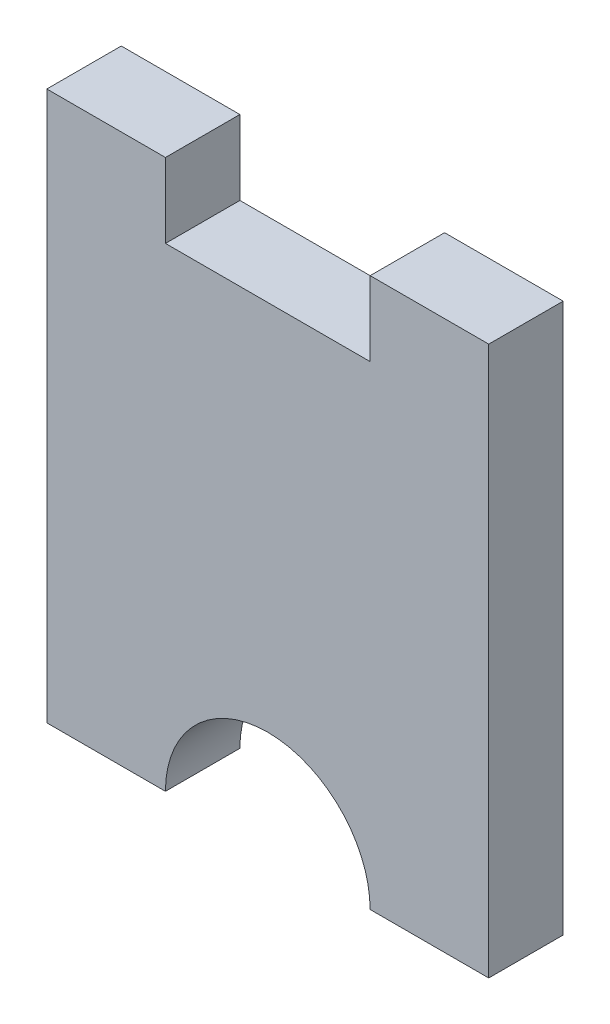
from build123d import *

# Parameters (mm, degrees)
BOSS_EXTRUDE1_DEPTH = 8


with BuildPart() as part:
    # Sketch1 → Boss-Extrude1 (new body)
    with BuildSketch(Plane.XY):
        with BuildLine():
            Line((-194.542584235, 40.149199278), (-207.290309428, 40.149199278))
            ThreePointArc((-207.290309428, 40.149199278), (-218.290309428, 51.149199278), (-229.290309428, 40.149199278))
            Line((-229.290309428, 40.149199278), (-242.038034621, 40.149199278))
            Line((-242.038034621, 40.149199278), (-242.038034621, 99.149199278))
            Line((-242.038034621, 99.149199278), (-229.288034621, 99.149199278))
            Line((-229.288034621, 99.149199278), (-229.288034621, 91.149199278))
            Line((-229.288034621, 91.149199278), (-207.288034621, 91.149199278))
            Line((-207.288034621, 91.149199278), (-207.288034621, 99.149199278))
            Line((-207.288034621, 99.149199278), (-194.542584235, 99.149199278))
            Line((-194.542584235, 99.149199278), (-194.542584235, 40.149199278))
        make_face()
    extrude(amount=BOSS_EXTRUDE1_DEPTH)


solid = part.part
